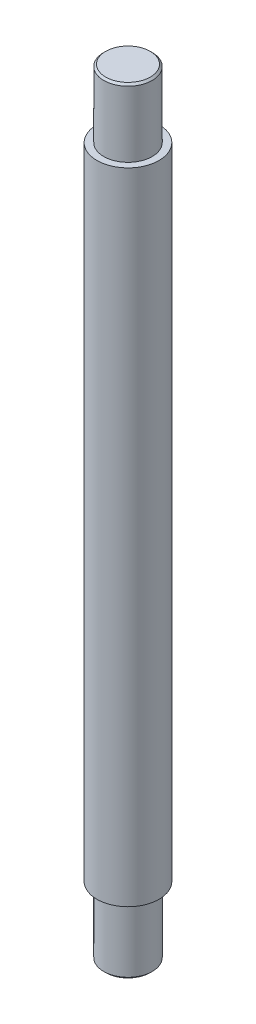
SolidWorks part; units mm, degrees
material "Q235B"
ref_plane "Front Plane" through (0, 0, 0) normal (0, 0, 1) x (1, 0, 0)
ref_plane "Top Plane" through (0, 0, 0) normal (0, 1, 0) x (1, 0, 0)
ref_plane "Right Plane" through (0, 0, 0) normal (1, 0, 0) x (0, 0, -1)
sketch "Sketch1" plane through (0, 0, 0) normal (0, 0, 1) x (1, 0, 0)
  line L0 (0, 0) -> (12.5, 0)
  line L1 (12.5, 0) -> (12.5, 35)
  line L2 (12.5, 35) -> (16, 35)
  line L3 (16, 35) -> (16, 365)
  line L4 (16, 365) -> (12.5, 365)
  line L5 (12.5, 365) -> (12.5, 400)
  line L6 (12.5, 400) -> (0, 400)
  line L7 (0, 400) -> (0, 0) construction
  line L8 (0, 0) -> (0, 400)
  dimension "D1" = 25
  dimension "D2" = 32
  dimension "D3" = 25
  dimension "D4" = 35
  dimension "D5" = 330
  dimension "D6" = 35
revolve "Revolve1" add sketch "Sketch1" angle 360 about L7
chamfer "Chamfer1" distance 1 angle 45 2 edges at (-12.5, 0, 0) (-12.5, 400, 0)
